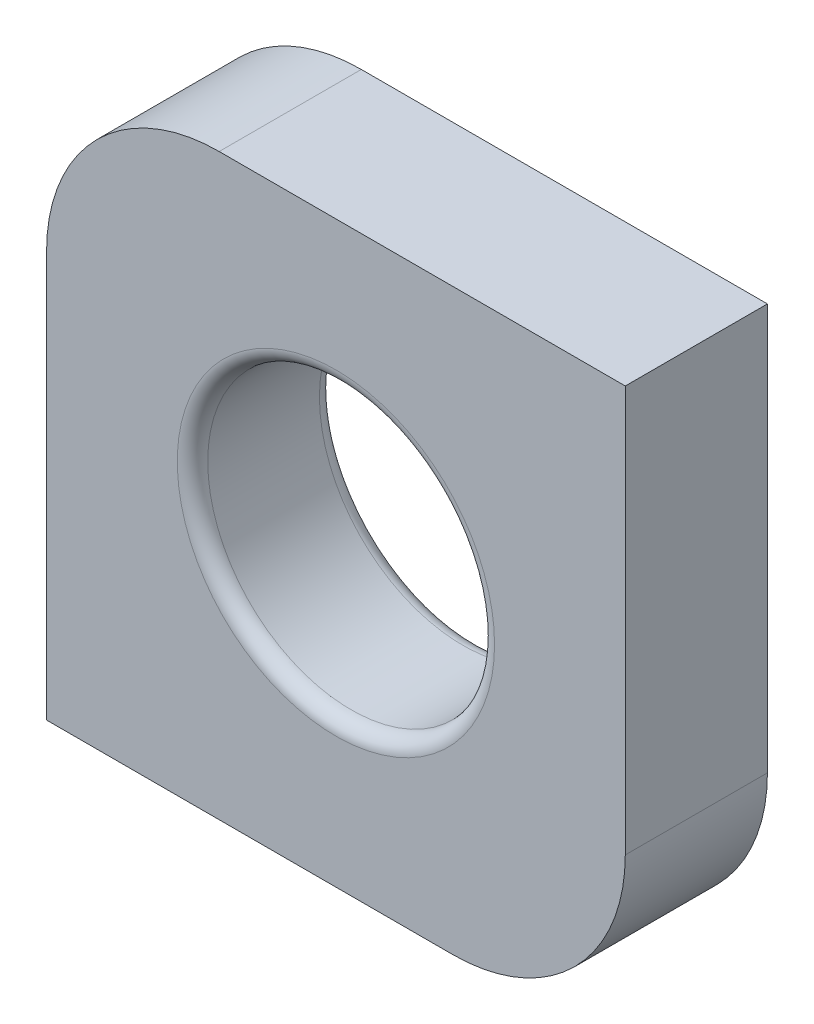
SolidWorks part; units mm, degrees
material "Plain Carbon Steel"
ref_plane "Front Plane" through (0, 0, 0) normal (0, 0, 1) x (1, 0, 0)
ref_plane "Top Plane" through (0, 0, 0) normal (0, 1, 0) x (1, 0, 0)
ref_plane "Right Plane" through (0, 0, 0) normal (1, 0, 0) x (0, 0, -1)
sketch "Sketch1" plane through (0, 0, 0) normal (0, 0, 1) x (1, 0, 0)
  line L0 (0, -2807.2089) -> (0, 137553.2352) construction
  line L1 (-2807.2089, 0) -> (137553.2352, 0) construction
  line L3 (-57, 57) -> (57, 57)
  line L4 (-57, 57) -> (-57, -57)
  line L5 (-57, -57) -> (57, -57)
  line L6 (57, 57) -> (57, -57)
  circle A0 centre (0, 0) radius 28.25
  dimension "D3" = 56.5
  dimension "D1" = 114
  dimension "D2" = 114
extrude "Boss-Extrude1" add sketch "Sketch1" along normal blind 28
fillet "Fillet1" radius 3 2 edges at (28.25, 0, 0) (28.25, 0, 28)
fillet "Fillet3" radius 34 2 edges at (57, -57, 14) (-57, 57, 14)
